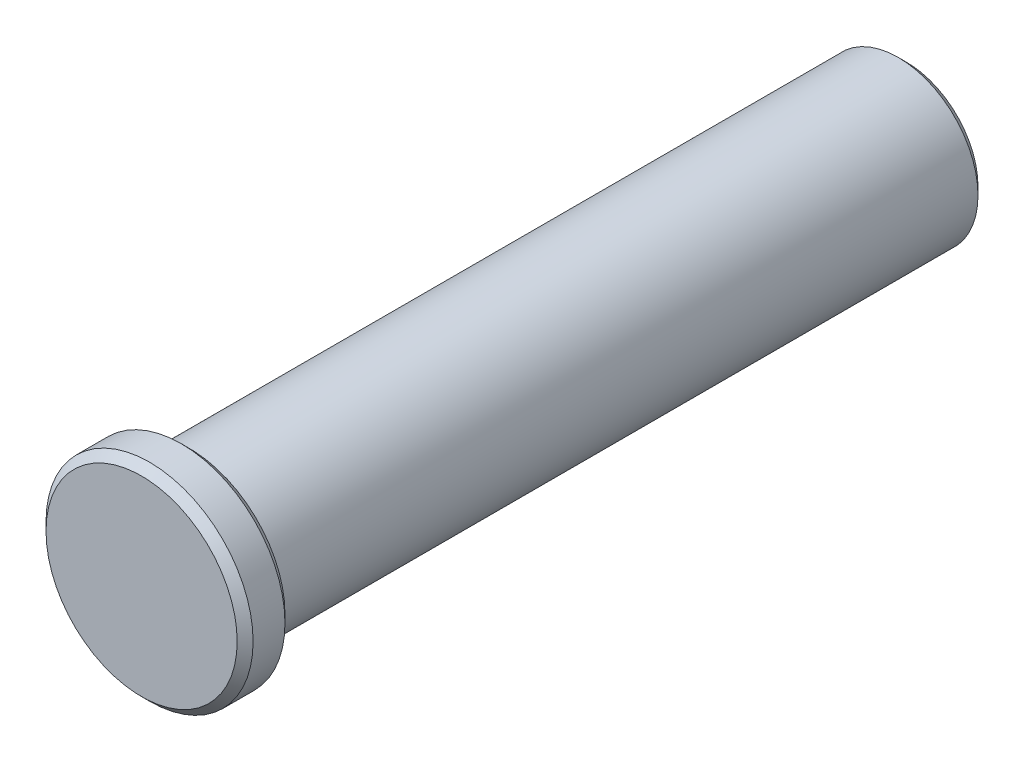
from build123d import *

# Parameters (mm, degrees)
SKETCH1_R           = 5
BOSS_EXTRUDE1_DEPTH = 45
SKETCH2_R           = 6.5
BOSS_EXTRUDE2_DEPTH = 3
CHAMFER1_SIZE       = 0.5


with BuildPart() as part:
    # Sketch1 → Boss-Extrude1 (new body)
    with BuildSketch(Plane.XY):
        with Locations(Location((0, 0, 0), (0, 0, 180))):
            Circle(SKETCH1_R)
    extrude(amount=BOSS_EXTRUDE1_DEPTH)

    # Sketch2 → Boss-Extrude2 (add)
    with BuildSketch(Plane.XY.offset(45)):
        Circle(SKETCH2_R)
    extrude(amount=BOSS_EXTRUDE2_DEPTH)

    # Chamfer1
    chamfer1_edges = [part.edges().sort_by_distance(p)[0] for p in [
        (5, 0, 0),
        (-6.5, 0, 45),
        (-6.5, 0, 48),
    ]]
    chamfer(chamfer1_edges, length=CHAMFER1_SIZE)


solid = part.part
